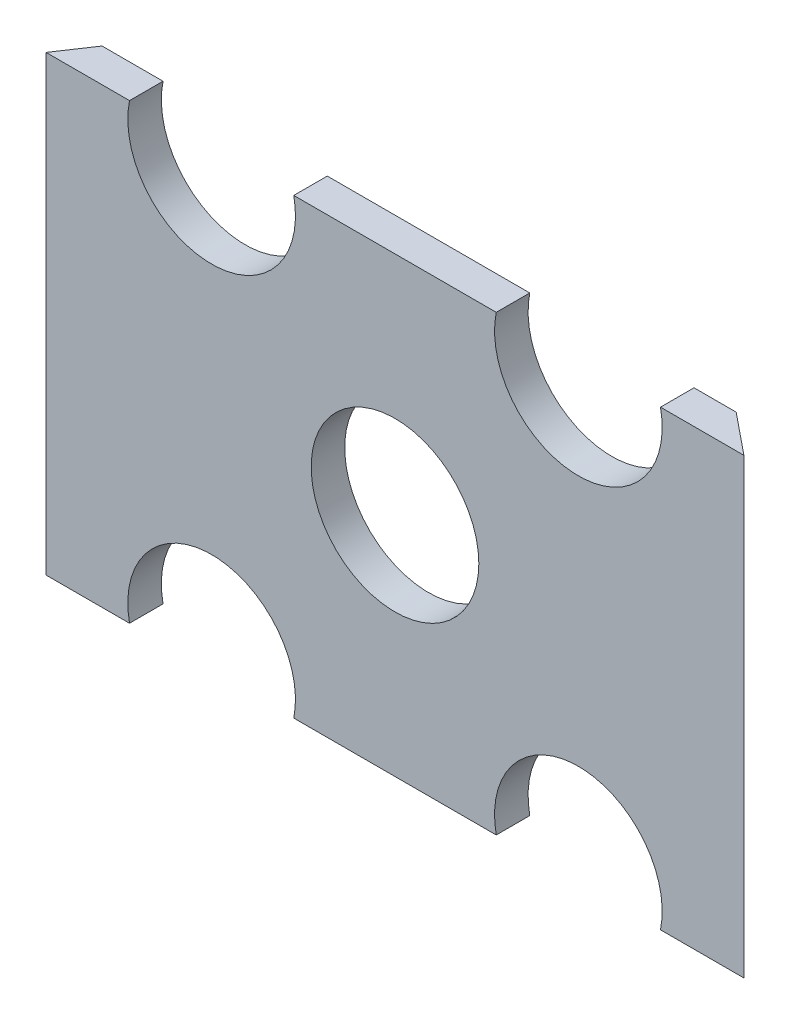
from build123d import *

# Parameters (mm, degrees)
SKETCH1_R           = 40
BOSS_EXTRUDE1_DEPTH = 16
CUT_EXTRUDE1_DEPTH  = 398.241740002


with BuildPart() as part:
    # Sketch1 → Boss-Extrude1 (new body)
    with BuildSketch(Plane.XY):
        with BuildLine():
            Line((0, 0), (39.808164115, 0))
            ThreePointArc((39.808164115, 0), (79, 48), (118.191835885, 0))
            Line((118.191835885, 0), (214.808164115, 0))
            ThreePointArc((214.808164115, 0), (254, 48), (293.191835885, 0))
            Line((293.191835885, 0), (333, 0))
            Line((333, 0), (333, 216))
            Line((333, 216), (293.191835885, 216))
            ThreePointArc((293.191835885, 216), (254, 168), (214.808164115, 216))
            Line((214.808164115, 216), (118.191835885, 216))
            ThreePointArc((118.191835885, 216), (79, 168), (39.808164115, 216))
            Line((39.808164115, 216), (0, 216))
            Line((0, 216), (0, 0))
        make_face()
        with Locations((166.5, 108)):
            Circle(SKETCH1_R, mode=Mode.SUBTRACT)
    extrude(amount=BOSS_EXTRUDE1_DEPTH)

    # Sketch2 → Cut-Extrude1 (cut, through all)
    with BuildSketch(Plane.XZ):
        Polygon((0, 16), (10.7, 0), (0, 0), align=None)
        Polygon((333, 16), (313.3, 0), (333, 0), align=None)
    extrude(amount=-CUT_EXTRUDE1_DEPTH, mode=Mode.SUBTRACT)


solid = part.part
